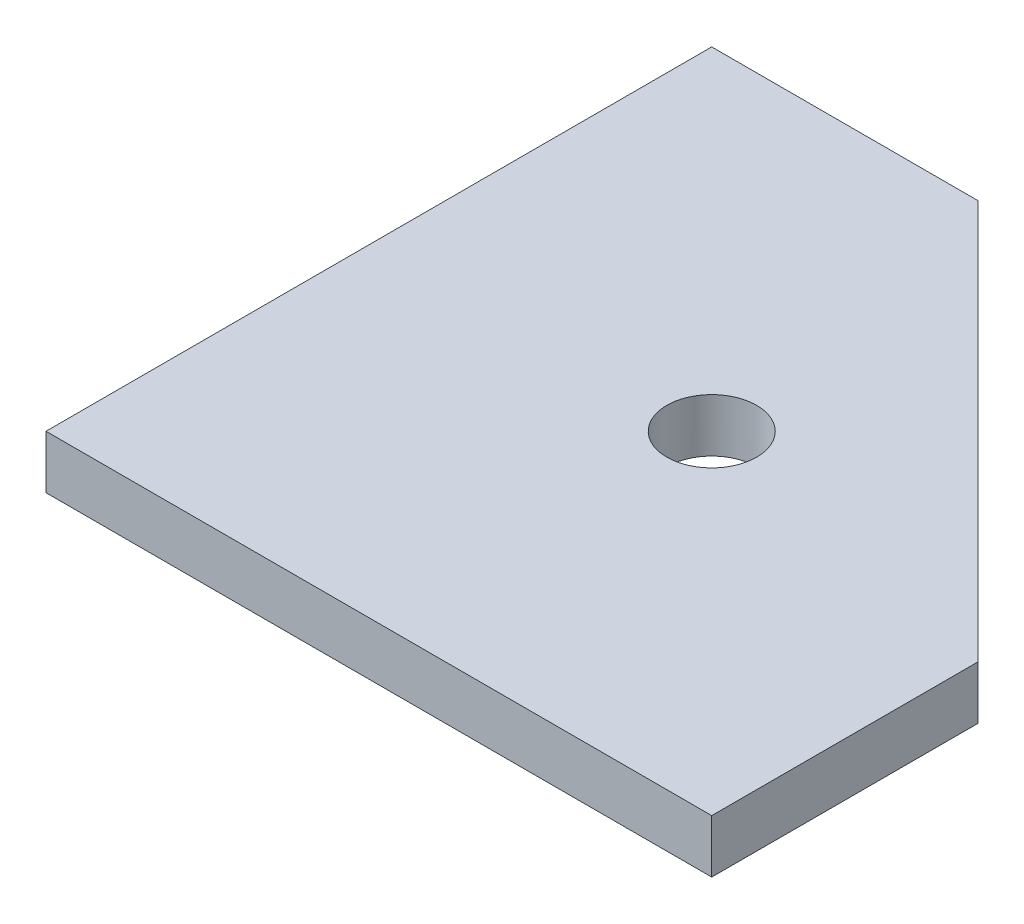
SolidWorks part; units mm, degrees
material "Q235"
ref_plane "Front" through (0, 0, 0) normal (0, 0, 1) x (1, 0, 0)
ref_plane "Top" through (0, 0, 0) normal (0, 1, 0) x (1, 0, 0)
ref_plane "Right" through (0, 0, 0) normal (1, 0, 0) x (0, 0, -1)
sketch "Sketch1" plane through (0, 0, 0) normal (0, 1, 0) x (1, 0, 0)
  line L1 (0, 0) -> (100, 0)
  line L2 (0, 0) -> (0, 100)
  line L3 (0, 100) -> (40, 100)
  line L5 (100, 0) -> (100, 40)
  line L6 (40, 100) -> (100, 40)
extrude "Boss-Extrude1" add sketch "Sketch1" along normal blind 8
hole_wizard "M12 Clearance Hole1" positions "Sketch5" profile "Sketch6" hole size "M12" standard "GB"
sketch "Sketch5" plane through (0, 8, 0) normal (0, 1, 0) x (1, 0, 0)
  line L0 (0, 0) -> (100, 0) construction
  line L1 (0, 100) -> (0, 0) construction
  point P0 (50, 50)
  dimension "D1" = 50
  dimension "D2" = 50
sketch "Sketch6" plane through (50, 8, -50) normal (1, 0, 0) x (0, 0, 1)
  line L0 (0, 0) -> (0, 64.0558)
  line L1 (0, 64.0558) -> (6.75, 60)
  line L2 (6.75, 60) -> (6.75, 0)
  line L5 (6.75, 0) -> (0, 0)
  line L10 (0, 64.0558) -> (-6.75, 60) construction
  line L11 (0, -6.35) -> (0, 107.95) construction
  dimension "孔直径" = 13.5
  dimension "孔深度" = 60
  dimension "导头角度" = 118
equation "\"D3@Sketch1\"=\"D1@Sketch1\""
